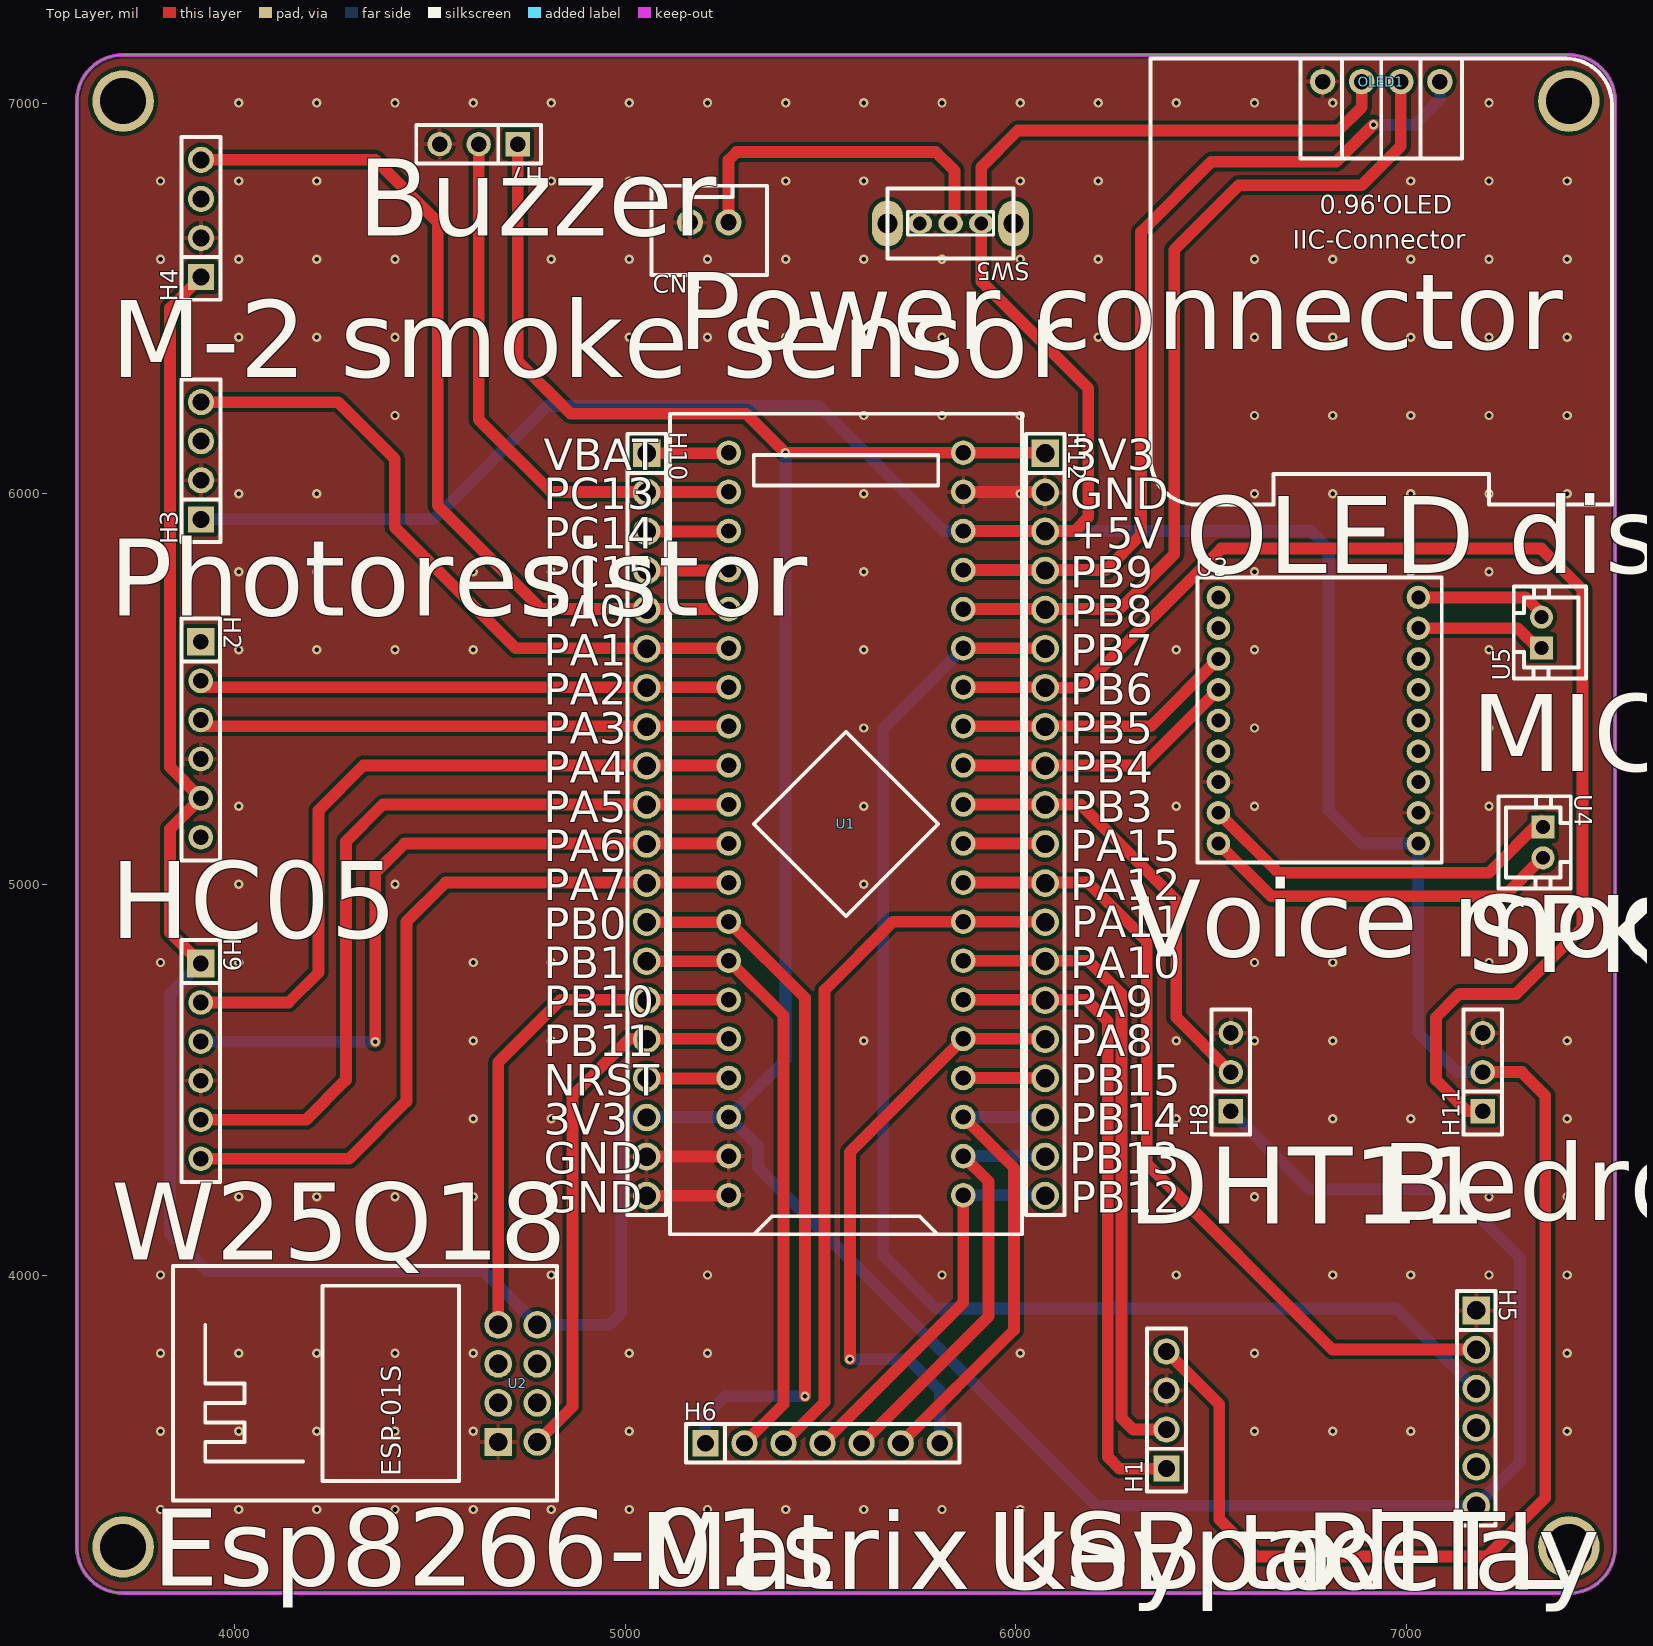
[diagram p0: Top Layer view]
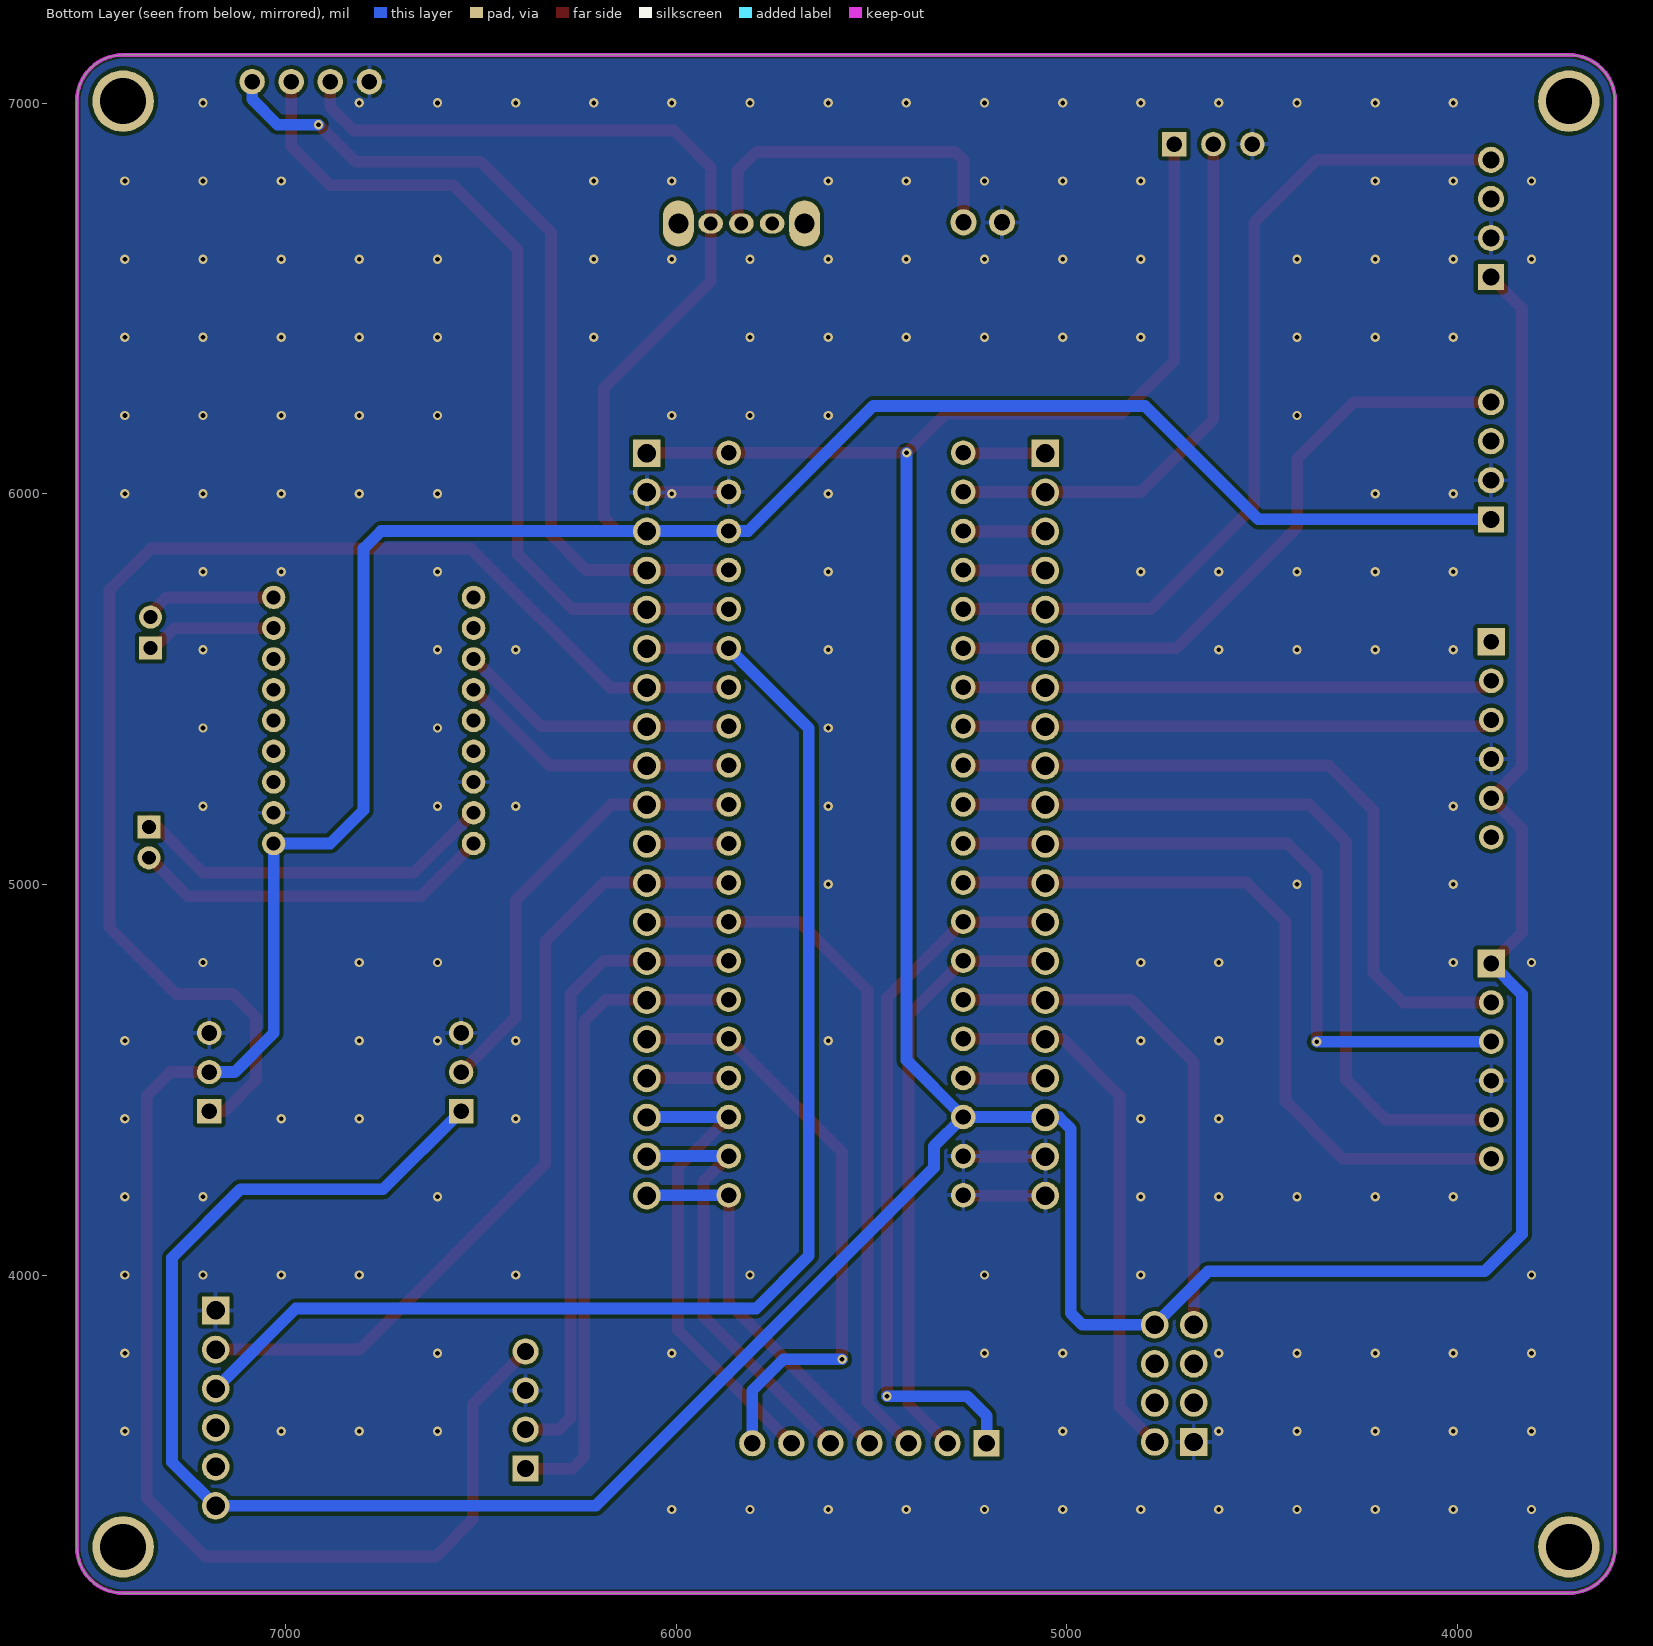
[diagram p1: Bottom Layer view, seen from below]
# Altium PCB MISC49851.pcbdoc
Units mil, origin at the board's own origin, x right, y up, seen from the top; angles counter-clockwise.
Board outline 3937.01 x 3937.01 mil, 2 copper layers (Top Layer, Bottom Layer), stack 62.206 mil thick; 20 components, 42 nets, 171 pads, 181 vias.

## Layer stack, top to bottom
Top Solder Mask Layer: solder mask 0.394, Dk 3.3
Top Layer: signal copper 1.379
Dielectric1: surface 59.449, FR4, Dk 4.5
Bottom Layer: signal copper 1.378
Bottom Solder Mask Layer: solder mask 0.394, Dk 3.3

## Board outline
3714.61,7123.5 ccw(c3714.61,7005.39) 3596.5,7005.39 3596.5,3304.61 ccw(c3714.61,3304.61) 3714.61,3186.5 7415.39,3186.5 ccw(c7415.39,3304.61) 7533.5,3304.61 7533.5,7005.39 ccw(c7415.39,7005.39) 7415.39,7123.5 3714.61,7123.5

## Design rules (kind name [scope] priority, off if disabled: settings)
BoardOutlineClearance copperThickness2oz_1 [All] p2 off: genericclearance=7.99 ignorepadtopadclearanceinfootprint=FALSE except(0: Arc-SplitContinuation Track-SplitContinuation SMDPad-SplitContinuation THPad-SplitContinuation Via-SplitContinuation Fill-SplitContinuation Region-SplitContinuation Poly-SplitContinuation Text-SplitContinuation Hole-SplitContinuation; 5.98: Arc-CutoutEdge Track-CutoutEdge SMDPad-CutoutEdge THPad-CutoutEdge Via-CutoutEdge Text-CutoutEdge; 6.9: Hole-OutlineEdge Hole-CutoutEdge; 10: Poly-OutlineEdge Poly-CutoutEdge; 11.81: Arc-OutlineEdge Track-OutlineEdge SMDPad-OutlineEdge THPad-OutlineEdge Via-OutlineEdge Fill-OutlineEdge Region-OutlineEdge Text-OutlineEdge Fill-CutoutEdge Region-CutoutEdge)
BoardOutlineClearance Plane_innerPlane_1 [All] p4 off: genericclearance=4.02 ignorepadtopadclearanceinfootprint=FALSE except(0: Arc-SplitContinuation Track-SplitContinuation SMDPad-SplitContinuation THPad-SplitContinuation Via-SplitContinuation Fill-SplitContinuation Region-SplitContinuation Poly-SplitContinuation Text-SplitContinuation Hole-SplitContinuation; 5.98: Arc-CutoutEdge Track-CutoutEdge SMDPad-CutoutEdge THPad-CutoutEdge Via-CutoutEdge Text-CutoutEdge; 6.9: Hole-OutlineEdge Hole-CutoutEdge; 10: Poly-OutlineEdge Poly-CutoutEdge; 11.81: Arc-OutlineEdge Track-OutlineEdge SMDPad-OutlineEdge THPad-OutlineEdge Via-OutlineEdge Fill-OutlineEdge Region-OutlineEdge Text-OutlineEdge Fill-CutoutEdge Region-CutoutEdge)
BoardOutlineClearance Copper_copperRegion_1 [All] p6 off: genericclearance=4.02 ignorepadtopadclearanceinfootprint=FALSE except(0: Arc-SplitContinuation Track-SplitContinuation SMDPad-SplitContinuation THPad-SplitContinuation Via-SplitContinuation Fill-SplitContinuation Region-SplitContinuation Poly-SplitContinuation Text-SplitContinuation Hole-SplitContinuation; 5.98: Arc-CutoutEdge Track-CutoutEdge SMDPad-CutoutEdge THPad-CutoutEdge Via-CutoutEdge Text-CutoutEdge; 6.9: Hole-OutlineEdge Hole-CutoutEdge; 10: Poly-OutlineEdge Poly-CutoutEdge; 11.81: Arc-OutlineEdge Track-OutlineEdge SMDPad-OutlineEdge THPad-OutlineEdge Via-OutlineEdge Fill-OutlineEdge Region-OutlineEdge Text-OutlineEdge Fill-CutoutEdge Region-CutoutEdge)
BoardOutlineClearance copperThickness1oz_1 [All] p8: genericclearance=4.02 ignorepadtopadclearanceinfootprint=FALSE except(0: Arc-SplitContinuation Track-SplitContinuation SMDPad-SplitContinuation THPad-SplitContinuation Via-SplitContinuation Fill-SplitContinuation Region-SplitContinuation Poly-SplitContinuation Text-SplitContinuation Hole-SplitContinuation; 5.98: Arc-CutoutEdge Track-CutoutEdge SMDPad-CutoutEdge THPad-CutoutEdge Via-CutoutEdge Text-CutoutEdge; 6.9: Hole-OutlineEdge Hole-CutoutEdge; 10: Poly-OutlineEdge Poly-CutoutEdge; 11.81: Arc-OutlineEdge Track-OutlineEdge SMDPad-OutlineEdge THPad-OutlineEdge Via-OutlineEdge Fill-OutlineEdge Region-OutlineEdge Text-OutlineEdge Fill-CutoutEdge Region-CutoutEdge)
Clearance copperThickness2oz [All] p1 off: gap=7.99 ignorepadtopadclearanceinfootprint=FALSE except(5.98: SMDPad-Track SMDPad-SMDPad THPad-Track SMDPad-THPad THPad-THPad Track-Via SMDPad-Via THPad-Via Via-Via Fill-SMDPad Region-SMDPad Fill-THPad Region-THPad Fill-Via Region-Via Fill-Fill Fill-Region Region-Region Arc-Track Arc-SMDPad Arc-THPad Arc-Via Fill-Arc Region-Arc Arc-Arc Text-Track SMDPad-Text Text-THPad Text-Via Fill-Text Region-Text Arc-Text Text-Text; 6.9: Hole-Track Hole-SMDPad Hole-THPad Hole-Via Fill-Hole Region-Hole Hole-Arc Hole-Text; 10: Poly-Track Poly-SMDPad Poly-THPad Poly-Via Poly-Fill Poly-Region Poly-Poly Poly-Arc Poly-Text Poly-Hole; 11.81: Fill-Track Region-Track)
Clearance Plane_innerPlane [All] p3 off: gap=4.02 ignorepadtopadclearanceinfootprint=FALSE except(5.98: SMDPad-Track SMDPad-SMDPad THPad-Track SMDPad-THPad THPad-THPad Track-Via SMDPad-Via THPad-Via Via-Via Fill-SMDPad Region-SMDPad Fill-THPad Region-THPad Fill-Via Region-Via Fill-Fill Fill-Region Region-Region Arc-Track Arc-SMDPad Arc-THPad Arc-Via Fill-Arc Region-Arc Arc-Arc Text-Track SMDPad-Text Text-THPad Text-Via Fill-Text Region-Text Arc-Text Text-Text; 6.9: Hole-Track Hole-SMDPad Hole-THPad Hole-Via Fill-Hole Region-Hole Hole-Arc Hole-Text; 10: Poly-Track Poly-SMDPad Poly-THPad Poly-Via Poly-Fill Poly-Region Poly-Poly Poly-Arc Poly-Text Poly-Hole; 11.81: Fill-Track Region-Track)
Clearance Copper_copperRegion [All] p5 off: gap=4.02 ignorepadtopadclearanceinfootprint=FALSE except(5.98: SMDPad-Track SMDPad-SMDPad THPad-Track SMDPad-THPad THPad-THPad Track-Via SMDPad-Via THPad-Via Via-Via Fill-SMDPad Region-SMDPad Fill-THPad Region-THPad Fill-Via Region-Via Fill-Fill Fill-Region Region-Region Arc-Track Arc-SMDPad Arc-THPad Arc-Via Fill-Arc Region-Arc Arc-Arc Text-Track SMDPad-Text Text-THPad Text-Via Fill-Text Region-Text Arc-Text Text-Text; 6.9: Hole-Track Hole-SMDPad Hole-THPad Hole-Via Fill-Hole Region-Hole Hole-Arc Hole-Text; 10: Poly-Track Poly-SMDPad Poly-THPad Poly-Via Poly-Fill Poly-Region Poly-Poly Poly-Arc Poly-Text Poly-Hole; 11.81: Fill-Track Region-Track)
Clearance copperThickness1oz [All] p7: gap=4.02 ignorepadtopadclearanceinfootprint=FALSE except(5.98: SMDPad-Track SMDPad-SMDPad THPad-Track SMDPad-THPad THPad-THPad Track-Via SMDPad-Via THPad-Via Via-Via Fill-SMDPad Region-SMDPad Fill-THPad Region-THPad Fill-Via Region-Via Fill-Fill Fill-Region Region-Region Arc-Track Arc-SMDPad Arc-THPad Arc-Via Fill-Arc Region-Arc Arc-Arc Text-Track SMDPad-Text Text-THPad Text-Via Fill-Text Region-Text Arc-Text Text-Text; 6.9: Hole-Track Hole-SMDPad Hole-THPad Hole-Via Fill-Hole Region-Hole Hole-Arc Hole-Text; 10: Poly-Track Poly-SMDPad Poly-THPad Poly-Via Poly-Fill Poly-Region Poly-Poly Poly-Arc Poly-Text Poly-Hole; 11.81: Fill-Track Region-Track)
DiffPairsRouting differentialPair [All] p1: maxlimit=6 minlimit=6 mostfreqgap=6 toplayer_minwidth=5 toplayer_prefwidth=10 toplayer_maxwidth=100 toplayer_mingap=6 toplayer_prefgap=6 toplayer_maxgap=6 bottomlayer_minwidth=5 bottomlayer_prefwidth=10 bottomlayer_maxwidth=100 bottomlayer_mingap=6 bottomlayer_prefgap=6 bottomlayer_maxgap=6 maxuncoupledlength=10
HoleToHoleClearance otherClearance [All] p1: gap=11.81 allowstackedmicrovias=TRUE
Length netLength [All] p1: minlimit=0 maxlimit=0
PasteMaskExpansion pasteMaskExpansion [All] p1: expansion=0
PlaneConnect innerPlane [All] p1: planeconnectstyle=Relief reliefexpansion=20 reliefentries=4 reliefconductorwidth=10 reliefairgap=10
PolygonConnect copperRegion [All] p1: connectstyle=Relief reliefconductorwidth=10 reliefentries=4 polygonreliefangle="90 Angle" airgapwidth=10 via.connectstyle=Relief via.reliefconductorwidth=10 via.reliefentries=4 via.polygonreliefangle="90 Angle" via.airgapwidth=10
RoutingVias viaSize [All] p1: holewidth=12.01 width=24.02 viastyle="Through Hole" minholewidth=11.81 minwidth=19.68 maxholewidth=248.03 maxwidth=393.7
SolderMaskExpansion solderMaskExpansion [IsVia] p1: expansion=-1000 istentingtop=TRUE
SolderMaskExpansion solderMaskExpansion [All] p2: expansion=2 istentingtop=FALSE
Width copperThickness2oz_2 [All] p1 off: maxlimit=100 minlimit=8 preferedwidth=10
Width copperThickness1oz_2 [All] p2: maxlimit=100 minlimit=5 preferedwidth=10

## Components (designator, comment, footprint, x,y, rotation, side; value= is the part's Value field where it differs from the comment)
CN4 "XH2.54*2P_THT" CONN-TH_2P-P2.50-XH2.54-2P 5215,6695 r0 top
H1 "" HDR-TH_4P-P2.54-V-F 6385,3655 r90 top
H2 "" HDR-TH_6P-P2.54-V-F 3913.62,5371.28 r270 top
H3 "" HDR-TH_4P-P2.54-V-F 3914.41,6084.75 r90 top
H4 "" HDR-TH_4P-P2.54-V-F 3914.41,6705 r90 top
H5 "" HDR-TH_6P-P2.54-V-M-1 7178.28,3659.9 r270 top
H6 "" HDR-TH_7P-P2.54-V-M 5505,3570 r0 top
H7 "" HDR-TH_3P-P2.54-V-F 4625,6895 r180 top
H8 "" HDR-TH_3P-P2.54-V-F 6550,4520 r90 top
H9 "" HDR-TH_6P-P2.54-V-F 3913.62,4548.18 r270 top
H10 "" HDR-TH_20P-P2.54-V-M-1 5054.9,5153.84 r270 top
H11 "" HDR-TH_3P-P2.54-V-F 7194.74,4520 r90 top
H12 "" HDR-TH_20P-P2.54-V-M-1 6074.58,5153.84 r270 top
OLED1 "" 0.96OLED_4P 6935,7055 r0 top
SW5 "" 拨动开关 5837.9,6692.05 r180 top
U1 "STM32F103C8T6-Card" CONN-TH_L53.3-W22.9_STM32F103C8T6-CARD 5565,5155 r90 top
U2 "ESP-01S" WIFIM-TH_ESP-01S 4725,3723.21 r90 top
U3 "CON2.0MM-PAD-18" CONN-TH_18P-P2.00_C9900078766 7030,5420 r90 top
U4 "PH2.0-2P" CONN-TH_2P-P2.00_BOSSIE_BX-PH2.0-2PZZ 7349.07,5107.81 r270 top
U5 "PH2.0-2P" CONN-TH_2P-P2.00_BOSSIE_BX-PH2.0-2PZZ 7345,5645 r90 top

## Footprints (in the part's own frame and the unit in brackets; to place one, negate y for a bottom-side part, rotate by r counter-clockwise, add the part's x,y. Pads: shape width x height; smd on the part's side, far side on the other; paste and mask are expansions set on the pad)
0.96OLED_4P [mm]
  round 1.65 hole 1 copper offset 0,0: 1(-3.81,-0.001) 2(-1.27,0.002) 3(1.27,0.002) 4(3.81,0.002)
  silkscreen extent -15,-27.5 15,1.5
CONN-TH_2P-P2.00_BOSSIE_BX-PH2.0-2PZZ [mm]
  rect 1.5x1.5 hole 0.9 paste+0 mask+0.05: 1(-1,0)
  round 1.5 hole 0.9 paste+0 mask+0.05: 2(1,0)
  silkscreen extent -3,-2.9 3,1.8
CONN-TH_2P-P2.50-XH2.54-2P [mm]
  round 1.7 hole 1.05 paste+0 mask+0.05: 1(1.25,0) 2(-1.25,0)
  silkscreen extent -3.75,-3.42 3.75,2.37
CONN-TH_18P-P2.00_C9900078766 [mil]
  round 60 hole 35.43 paste+0 mask+1.97: 1(-314.96,0.01) 2(-314.96,511.81) 3(-236.22,0.01) 4(-236.22,511.81) 5(-157.48,0.01) 6(-157.48,511.81) 9(0,0) 10(0,511.81) 11(78.74,0) 12(78.74,511.81) 13(157.48,0) 14(157.48,511.81) 15(236.22,0) 16(236.22,511.81) 17(314.96,0) 18(314.96,511.81)
  round 60 hole 35.43 copper offset -0.01,0 paste+0 mask+1.97: 7(-78.72,0.01) 8(-78.72,511.81)
  silkscreen extent -363,-60 365,565
CONN-TH_L53.3-W22.9_STM32F103C8T6-CARD [mm]
  round 1.6 hole 1: 1(-24.13,-7.62) 2(-21.59,-7.62) 3(-19.05,-7.62) 4(-16.51,-7.62) 5(-13.97,-7.62) 6(-11.43,-7.62) 7(-8.89,-7.62) 8(-6.35,-7.62) 9(-3.81,-7.62) 10(-1.27,-7.62) 11(1.27,-7.62) 12(3.81,-7.62) 13(6.35,-7.62) 14(8.89,-7.62) 15(11.43,-7.62) 16(13.97,-7.62) 17(16.51,-7.62) 18(19.05,-7.62) 19(21.59,-7.62) 20(24.13,-7.62) 21(24.13,7.62) 22(21.59,7.62) 23(19.05,7.62) 24(16.51,7.62) 25(13.97,7.62) 26(11.43,7.62) 27(8.89,7.62) 28(6.35,7.62) 29(3.81,7.62) 30(1.27,7.62) 31(-1.27,7.62) 32(-3.81,7.62) 33(-6.35,7.62) 34(-8.89,7.62) 35(-11.43,7.62) 36(-13.97,7.62) 37(-16.51,7.62) 38(-19.05,7.62) 39(-21.59,7.62) 40(-24.13,7.62)
  silkscreen extent -26.67,-11.43 26.67,11.43
HDR-TH_3P-P2.54-V-F [mil]
  rect 62x62 hole 40.16: 1(-100,0)
  round 62 hole 40.16: 2(0,0) 3(100,0)
  silkscreen extent -160,-49 160,49
HDR-TH_4P-P2.54-V-F [mm]
  rect 1.7x1.7 hole 1.1: 1(-3.81,0)
  round 1.7 hole 1.1: 2(-1.27,0) 3(1.27,0) 4(3.81,0)
  silkscreen extent -5.29,-1.27 5.29,1.27
HDR-TH_6P-P2.54-V-F [mm]
  rect 1.8x1.8 hole 1.02: 1(-6.35,0)
  round 1.6 hole 1.02: 2(-3.81,0) 3(-1.27,0) 4(1.27,0) 5(3.81,0) 6(6.35,0)
  silkscreen extent -7.87,-1.25 7.87,1.25
HDR-TH_6P-P2.54-V-M-1 [mm]
  rect 1.8x1.8 hole 1.2: 1(-6.35,0)
  round 1.8 hole 1.2: 2(-3.81,0) 3(-1.27,0) 4(1.27,0) 5(3.81,0) 6(6.35,0)
  silkscreen extent -7.62,-1.25 7.62,1.25
HDR-TH_7P-P2.54-V-M [mm]
  rect 1.7x1.7 hole 1.1: 1(-7.62,0)
  round 1.7 hole 1.1: 2(-5.08,0) 3(-2.54,0) 4(0,0) 5(2.54,0) 6(5.08,0) 7(7.62,0)
  silkscreen extent -8.89,-1.25 8.89,1.25
HDR-TH_20P-P2.54-V-M-1 [mm]
  rect 1.8x1.8 hole 1.2: 1(-24.13,0)
  round 1.8 hole 1.2: 2(-21.59,0) 3(-19.05,0) 4(-16.51,0) 5(-13.97,0) 6(-11.43,0) 7(-8.89,0) 8(-6.35,0) 9(-3.81,0) 10(-1.27,0) 11(1.27,0) 12(3.81,0) 13(6.35,0) 14(8.89,0) 15(11.43,0) 16(13.97,0) 17(16.51,0) 18(19.05,0) 19(21.59,0) 20(24.13,0)
  silkscreen extent -25.4,-1.25 25.4,1.25
WIFIM-TH_ESP-01S [mm]
  rect 1.8x1.8 hole 1.2: 1(-3.81,1.27)
  round 1.8 hole 1.2: 2(-1.27,1.27) 3(1.27,1.27) 4(3.81,1.27) 5(3.81,-1.27) 6(1.27,-1.27) 7(-1.27,-1.27) 8(-3.81,-1.27)
  silkscreen extent -7.62,-2.54 7.62,22.4
拨动开关 [mil]
  oval 63x51.2 hole 35.4 paste+0 mask+2: 1(-73.4,0) 2(5,0) 3(84,0)
  oval 78.7x118.1 hole 51.2 paste+0 mask+2: 4(166.7,0) 5(-156.1,0)
  silkscreen extent -156,-90 167,90

## Free pads (board coordinates)
  round 157.48 hole 118.11: 1(3714.61,7005.39) 1(3714.61,3304.61) 1(7415.39,7005.39) 1(7415.39,3304.61)

## Via types
v1: diameter 24.02, hole 12, Top Layer to Bottom Layer, 181 vias

## Nets (pads, with @x,y where several pads share a name; then routed paths per layer and width w, separated by ;. In a path a pad name is that pad's centre, name@x,y a point inside that pad or via, vN(x,y) a via of type N, cw(c..) or ccw(c..) an arc to the next point about the centre after c; other vN are vias at no path point)
$1N17118: CN4.1 SW5.2 | length 901.4
  Top Layer w30: CN4.1 5264.22,6854.22 5285,6875 5795,6875 5842.9,6827.1 SW5.2@5842.9,6692.05
+5V: H1.4 H3.1 H11.2 H12.3 OLED1.2 SW5.1 U1.18 U3.1 | length 9867.5
  Top Layer w30: U1.18 6150,5905 6185,5940 6185,6270 5911.3,6543.7 SW5.1 5911.3,6836.3 6005,6930 6825,6930 6885,6990 OLED1.2@6885,7055.05 ; H1.4 6520,3670 6520,3375 6615,3280 7205,3280 7355,3430 7355,4460 7295,4520 H11.2
  Bottom Layer w30: H3.1 4509.75,5934.75 4800,6225 5495,6225 5815,5905 U1.18 6755,5905 6800,5860 6800,5190 6884.96,5105.04 U3.1 7029.99,4620.01 7130,4520 H11.2
GND: CN4.2 H1.3 H2.4 H3.2 H4.2 H5.1 H7.3 H8.3 H9.4 H10.19 H10.20 H11.3 H12.2 OLED1.1 U1.19 U1.39 U1.40 U2.1 U3.3 U3.6 | length 631.2
  Top Layer w30: H10.20 5263.83,4203.84 U1.40 ; H10.19 5263.83,4303.84 U1.39 ; U1.19 6073.41,6005 H12.2
  other v1: 3810.6,3400.6 4010.6,3400.6 4210.6,3400.6 4410.6,3400.6 4610.6,3400.6 4810.6,3400.6 5010.6,3400.6 5210.6,3400.6 5410.6,3400.6 5610.6,3400.6 5810.6,3400.6 6010.6,3400.6 3810.6,3600.6 4010.6,3600.6 4210.6,3600.6 4410.6,3600.6 4610.6,3600.6 5010.6,3600.6 6610.6,3600.6 6810.6,3600.6 7010.6,3600.6 7410.6,3600.6 3810.6,3800.6 4010.6,3800.6 4210.6,3800.6 4410.6,3800.6 4610.6,3800.6 5010.6,3800.6 5210.6,3800.6 6010.6,3800.6 6610.6,3800.6 7410.6,3800.6 3810.6,4000.6 4810.6,4000.6 5210.6,4000.6 5810.6,4000.6 6410.6,4000.6 6810.6,4000.6 7010.6,4000.6 7210.6,4000.6 7410.6,4000.6 4010.6,4200.6 4210.6,4200.6 4410.6,4200.6 4610.6,4200.6 4810.6,4200.6 6610.6,4200.6 7210.6,4200.6 7410.6,4200.6 4610.6,4400.6 4810.6,4400.6 6410.6,4400.6 6810.6,4400.6 7010.6,4400.6 7410.6,4400.6 4610.6,4600.6 4810.6,4600.6 5610.6,4600.6 6410.6,4600.6 6610.6,4600.6 6810.6,4600.6 7410.6,4600.6 3810.6,4800.6 4010.6,4800.6 4610.6,4800.6 4810.6,4800.6 6610.6,4800.6 6810.6,4800.6 7210.6,4800.6 4010.6,5000.6 4410.6,5000.6 5610.6,5000.6 4010.6,5200.6 5610.6,5200.6 6410.6,5200.6 6610.6,5200.6 7210.6,5200.6 5610.6,5400.6 6610.6,5400.6 7210.6,5400.6 4010.6,5600.6 4210.6,5600.6 4410.6,5600.6 4610.6,5600.6 5610.6,5600.6 6410.6,5600.6 6610.6,5600.6 7210.6,5600.6 4010.6,5800.6 4210.6,5800.6 4410.6,5800.6 4610.6,5800.6 4810.6,5800.6 5610.6,5800.6 6610.6,5800.6 7010.6,5800.6 7210.6,5800.6 4010.6,6000.6 4210.6,6000.6 5610.6,6000.6 6010.6,6000.6 6610.6,6000.6 6810.6,6000.6 7010.6,6000.6 7210.6,6000.6 7410.6,6000.6 4410.6,6200.6 5610.6,6200.6 5810.6,6200.6 6010.6,6200.6 6610.6,6200.6 6810.6,6200.6 7010.6,6200.6 7210.6,6200.6 7410.6,6200.6 4010.6,6400.6 4210.6,6400.6 4410.6,6400.6 4810.6,6400.6 5010.6,6400.6 5210.6,6400.6 5410.6,6400.6 5610.6,6400.6 5810.6,6400.6 6210.6,6400.6 6610.6,6400.6 6810.6,6400.6 7010.6,6400.6 7210.6,6400.6 7410.6,6400.6 3810.6,6600.6 4010.6,6600.6 4210.6,6600.6 4410.6,6600.6 4810.6,6600.6 5010.6,6600.6 5210.6,6600.6 5410.6,6600.6 5610.6,6600.6 5810.6,6600.6 6010.6,6600.6 6210.6,6600.6 6610.6,6600.6 6810.6,6600.6 7010.6,6600.6 7210.6,6600.6 7410.6,6600.6 3810.6,6800.6 4010.6,6800.6 4210.6,6800.6 4810.6,6800.6 5010.6,6800.6 5210.6,6800.6 5410.6,6800.6 5610.6,6800.6 6010.6,6800.6 6210.6,6800.6 7010.6,6800.6 7210.6,6800.6 7410.6,6800.6 4010.6,7000.6 4210.6,7000.6 4410.6,7000.6 4610.6,7000.6 4810.6,7000.6 5010.6,7000.6 5210.6,7000.6 5410.6,7000.6 5610.6,7000.6 5810.6,7000.6 6010.6,7000.6 6210.6,7000.6 6410.6,7000.6 6610.6,7000.6 6810.6,7000.6 7210.6,7000.6
MIC+: U3.17 U5.2 | length 324.8
  Top Layer w30: U3.17 7304.26,5734.96 U5.2@7340,5699.22
MIC-: U3.15 U5.1 | length 333
  Top Layer w30: U3.15 7284.56,5656.22 U5.1@7340,5600.78
NRST: H10.17 U1.37 | length 210.6
  Top Layer w30: H10.17 5263.83,4503.84 U1.37
PA0: H4.4 H10.5 U1.25 | length 2251.6
  Top Layer w30: H4.4 4360,6855 4520,6695 4520,5970 4785,5705 U1.25
PA1: H3.4 H10.6 U1.26 | length 1714
  Top Layer w30: H3.4 4265.25,6234.75 4410,6090 4410,5915 4720,5605 U1.26
PA2: H2.2 H10.7 U1.27 | length 1358.1
  Top Layer w30: H2.2 3929.9,5505 U1.27
PA3: H2.3 H10.8 U1.28 | length 1358.1
  Top Layer w30: H2.3 3929.9,5405 U1.28
PA4: H9.2 H10.9 U1.29 | length 1845.8
  Top Layer w30: H9.2 4138.18,4698.18 4215,4775 4215,5190 4330,5305 U1.29
PA5: H9.5 H10.10 U1.30 | length 2042.9
  Top Layer w30: H9.5 4183.18,4398.18 4285,4500 4285,5110 4380,5205 U1.30
PA6: H9.3 H10.11 U1.31 | length 1814.8
  Top Layer w30: v1(4360,4597.78) 4360,5030 4435,5105 U1.31
  Bottom Layer w30: H9.3 3914.03,4597.78 v1(4360,4597.78)
PA7: H9.6 H10.12 U1.32 | length 1913.6
  Top Layer w30: H9.6 4293.18,4298.18 4440,4445 4440,4905 4540,5005 U1.32
PA8: H6.7 H12.16 U1.5 | length 1548.3
  Top Layer w30: v1(5575,3785) 5575,4315 U1.5 6073.41,4605 H12.16
  Bottom Layer w30: v1(5575,3785) 5725,3785 5805,3705 H6.7
PA9: H1.1 H12.15 U1.6 | length 1670.2
  Top Layer w30: U1.6 6180,4705 6235,4650 6235,3535 6265,3505 H1.1
PA10: H1.2 H12.14 U1.7 | length 1652.6
  Top Layer w30: U1.7 6185,4805 6270,4720 6270,3635 6300,3605 H1.2
PA11: H6.3 H12.13 U1.8 | length 1841
  Top Layer w30: H6.3 5510,3675 5510,4730 5685,4905 U1.8 6073.41,4905 H12.13
PA12: H5.2 H12.12 U1.9 | length 2142.2
  Top Layer w30: U1.9 6185,5005 6335,4855 6335,4285 6810.1,3809.9 H5.2
PA15: H12.11 U1.10 | length 210.1
  Top Layer w30: U1.10 6073.41,5105 H12.11
PB0: H6.1 H10.13 U1.33 | length 1852.1
  Top Layer w30: H10.13 5263.83,4903.84 U1.33 5460,4710 v1(5460,3690)
  Bottom Layer w30: H6.1 5205,3640 5255,3690 v1(5460,3690)
PB1: H6.2 H10.14 U1.34 | length 1545
  Top Layer w30: H10.14 5263.83,4803.84 U1.34 5405,4665 5405,3670 H6.2
PB3: H8.2 H12.10 U1.11 | length 1144.5
  Top Layer w30: U1.11 6165,5205 6410,4960 6410,4660 H8.2
PB4: H12.9 U1.12 U3.12 | length 733.4
  Top Layer w30: U1.12 6324.45,5305 U3.12
PB5: H12.8 U1.13 U3.14 | length 724.6
  Top Layer w30: U1.13 6345.71,5405 U3.14
PB6: H11.1 H12.7 U1.14 | length 3424.7
  Top Layer w30: U1.14 6073.41,5505 H12.7 6168.84,5503.84 6525,5860 7345,5860 7450,5755 7450,4890 7280,4720 7135,4720 7075,4660 7075,4500 7155,4420 H11.1
PB7: H5.3 H12.6 U1.15 | length 3509.1
  Top Layer w30: U1.15 6073.41,5605 H12.6
  Bottom Layer w30: U1.15 5660,5400 5660,4050 5795,3915 6973.18,3915 H5.3
PB8: H12.5 OLED1.3 U1.16 | length 2232.8
  Top Layer w30: U1.16 6265,5705 6405,5845 6405,6625 6570,6790 6885,6790 6985,6890 OLED1.3@6985,7055.05
PB9: H12.4 OLED1.4 U1.17 | length 2218.2
  Top Layer w30: U1.17 6230,5805 6320,5895 6320,6670 6500,6850 6820,6850 v1(6915,6945)
  Bottom Layer w30: v1(6915,6945) 7020,6945 7085,7010 OLED1.4@7085,7055.05
PB10: H10.15 U1.35 U2.4 | length 1328.1
  Top Layer w30: U2.4 4675,4545 4835,4705 U1.35
PB11: H10.16 U1.36 U2.8 | length 1384.1
  Top Layer w30: U2.8 4865,3663.21 4865,4460 5010,4605 U1.36
PB12: H6.4 H12.20 U1.1 | length 994.2
  Top Layer w30: H6.4 5865,3930 U1.1
  Bottom Layer w30: U1.1 6073.41,4205 H12.20
PB13: H6.5 H12.19 U1.2 | length 1106.6
  Top Layer w30: H6.5 5930,3895 5930,4240 U1.2
  Bottom Layer w30: U1.2 6073.41,4305 H12.19
PB14: H6.6 H12.18 U1.3 | length 1219
  Top Layer w30: H6.6 5995,3860 5995,4275 U1.3
  Bottom Layer w30: U1.3 6073.41,4405 H12.18
PB15: H12.17 U1.4 | length 210.1
  Top Layer w30: U1.4 6073.41,4505 H12.17
PC13: H7.2 H10.2 U1.22 | length 1421.6
  Top Layer w30: H7.2 4625,6190 4810,6005 U1.22
PC14: H10.3 U1.23 | length 210.6
  Top Layer w30: H10.3 5263.83,5903.84 U1.23
PC15: H10.4 U1.24 | length 210.6
  Top Layer w30: H10.4 5263.83,5803.84 U1.24
SPK+: U3.2 U4.2 | length 922.4
  Top Layer w30: U3.2 6653.23,4970 7249.22,4970 U4.2@7345,5065.78
SPK-: U3.4 U4.1 | length 946.1
  Top Layer w30: U3.4 6671.97,5030 7210.78,5030 U4.1@7345,5164.22
VBAT: H10.1 U1.21 | length 210.6
  Top Layer w30: H10.1 5263.83,6103.84 U1.21
VCC: H2.5 H4.1 H5.6 H7.1 H8.1 H9.1 H10.18 H12.1 U1.20 U1.38 U2.5 | length 12332.7
  Top Layer w30: H9.1 3835,4876.81 3835,5142.66 H2.5 3835,5299.91 3835,6475.59 H4.1 ; H7.1 4725,6340 4860,6205 5310,6205 v1(5410,6105) U1.20 6073.41,6105 H12.1
  Bottom Layer w30: H9.1 3835,4719.56 3835,4105 3930,4010 4638.21,4010 U2.5 4960,3873.21 4990,3903.21 4990,4375 5020,4405 U1.38 ; v1(5410,6105) 5410,4550 U1.38 ; H8.1 6750,4220 7115,4220 7290,4045 7290,3521.62 H5.6 6205.1,3409.9 5340,4275 5340,4330 U1.38
pads on no net: H2.1 H2.6 H3.3 H4.3 H5.4 H5.5 SW5.3 SW5.4 SW5.5 U2.2 U2.3 U2.6 U2.7 U3.5 U3.7 U3.8 U3.9 U3.10 U3.11 U3.13 U3.16 U3.18

## Polygon pours and split planes (outlines as drawn)
GND on Bottom Layer (solid, remove dead copper, pour order 2): 3525,7245 3525,3080 7700,3080 7700,7245
GND on Top Layer (solid, remove dead copper, pour order 2): 3000,7415 3000,3000 7930,3000 7930,7415

## Keep-outs
Board Outline Layer:
  the board outline again, w10

## Silkscreen, mask and mechanical layers (free items; w line width, h text height)
Top Silkscreen Layer:
  text "Design and Implementation of an STM32-Based Smart Home System" at 4180,6990 h118.11
  text "Buzzer" at 4315,6660 h196.85
  text "Power connector" at 5135,6370 h196.85
  text "M-2 smoke sensor" at 3682.62,6298.39 h196.85
  text "VBAT" at 4790.95,6060 h80
  text "3V3" at 6139.16,6060 h80
  text "PC13" at 4790.95,5960 h80
  text "GND" at 6139.16,5960 h80
  text "PC14" at 4790.95,5860 h80
  text "+5V" at 6139.16,5860 h80
  text "OLED display" at 6433.66,5796.57 h196.85
  text "PC15" at 4790.95,5760 h80
  text "PB9" at 6139.16,5760 h80
  text "Photoresistor" at 3679.64,5687.98 h196.85
  text "PA0" at 4790.95,5660 h80
  text "PB8" at 6139.16,5660 h80
  text "PA1" at 4790.95,5560 h80
  text "PB7" at 6139.16,5560 h80
  text "PA2" at 4790.95,5460 h80
  text "PB6" at 6139.16,5460 h80
  text "PA3" at 4790.95,5360 h80
  text "PB5" at 6139.16,5360 h80
  text "MIC" at 7165,5290 h196.85
  text "PA4" at 4790.95,5260 h80
  text "PB4" at 6139.16,5260 h80
  text "PA5" at 4790.95,5160 h80
  text "PB3" at 6139.16,5160 h80
  text "PA6" at 4790.95,5060 h80
  text "PA15" at 6139.16,5060 h80
  text "PA7" at 4790.95,4960 h80
  text "PA12" at 6139.16,4960 h80
  text "PA11" at 6140.95,4865 h80
  text "HC05" at 3681.43,4863.1 h196.85
  text "PB0" at 4790.95,4860 h80
  text "Voice module" at 6290,4815 h196.85
  text "SPK" at 7155,4775 h196.85
  text "PB1" at 4790.95,4760 h80
  text "PA10" at 6139.16,4760 h80
  text "PB10" at 4790.95,4660 h80
  text "PA9" at 6139.16,4660 h80
  text "PB11" at 4790.95,4560 h80
  text "PA8" at 6139.16,4560 h80
  text "NRST" at 4790.95,4460 h80
  text "PB15" at 6139.16,4460 h80
  text "3V3" at 4790.95,4360 h80
  text "PB14" at 6139.16,4360 h80
  text "GND" at 4790.95,4260 h80
  text "PB13" at 6135.95,4260 h80
  text "GND" at 4790.95,4160 h80
  text "PB12" at 6139.16,4160 h80
  text "Bedroom light" at 6935,4141.42 h196.85
  text "DHT11" at 6286.3,4131.57 h196.85
  text "W25Q18" at 3685,4040 h196.85
  text "Esp8266-01s" at 3790,3205 h196.85
  text "Matrix keypad" at 5035,3196.87 h196.85
  text "USB to TTL" at 5925.61,3196.57 h196.85
  text "Relay" at 6740,3195 h196.85